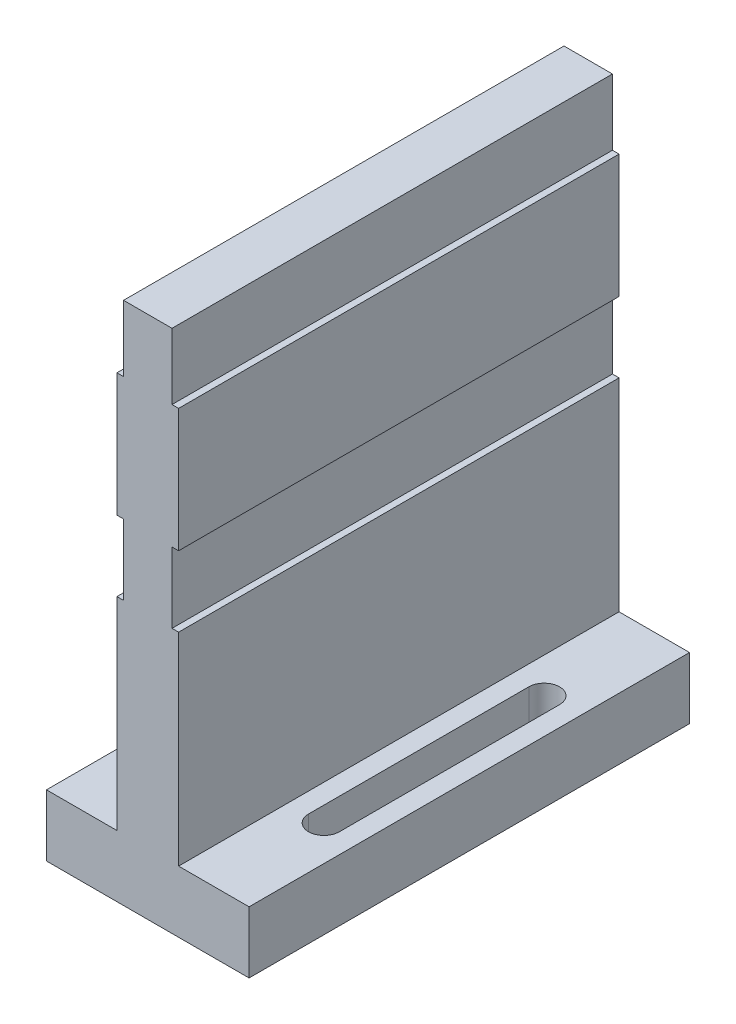
SolidWorks part; units mm, degrees
ref_plane "前视基准面" through (0, 0, 0) normal (0, 0, 1) x (1, 0, 0)
ref_plane "上视基准面" through (0, 0, 0) normal (0, 1, 0) x (1, 0, 0)
ref_plane "右视基准面" through (0, 0, 0) normal (1, 0, 0) x (0, 0, -1)
sketch "草图1" plane through (0, 0, 0) normal (0, 0, 1) x (1, 0, 0)
  line L0 (0, 0) -> (23, 0)
  line L1 (23, 0) -> (23, 14)
  line L2 (23, 14) -> (7, 14)
  line L3 (7, 14) -> (7, 119)
  line L4 (7, 119) -> (-7, 119)
  line L5 (-7, 119) -> (-7, 14)
  line L6 (-7, 14) -> (-23, 14)
  line L7 (-23, 14) -> (-23, 0)
  line L8 (-23, 0) -> (0, 0)
  dimension "D1" = 14
  dimension "D2" = 14
  dimension "D3" = 16
  dimension "D4" = 105
extrude "凸台-拉伸1" add sketch "草图1" along normal mid plane 100
sketch "草图2" plane through (0, 14, 0) normal (0, 1, 0) x (1, 0, 0)
  line L0 (15, -25) -> (15, 25) construction
  line L1 (11.5, -25) -> (11.5, 25)
  line L2 (18.5, -25) -> (18.5, 25)
  line L3 (23, -50) -> (23, 50) construction
  arc A0 (11.5, -25) -> (18.5, -25) centre (15, -25) ccw
  arc A1 (18.5, 25) -> (11.5, 25) centre (15, 25) ccw
  point P2 (15, 0)
  dimension "D3" = 3.5
  dimension "D1" = 50
  dimension "D2" = 8
extrude "切除-拉伸1" cut sketch "草图2" against normal up to next
sketch "草图3" plane through (7, 0, 0) normal (1, 0, 0) x (0, 0, -1)
  line L0 (50, 14) -> (50, 119) construction
  line L1 (-50, 119) -> (50, 119)
  line L2 (-50, 119) -> (-50, 104)
  line L3 (-50, 104) -> (50, 104)
  line L4 (50, 119) -> (50, 104)
  line L5 (-50, 14) -> (-50, 119) construction
  line L6 (-50, 76) -> (50, 76)
  line L7 (-50, 76) -> (-50, 60)
  line L8 (-50, 60) -> (50, 60)
  line L9 (50, 76) -> (50, 60)
  dimension "D1" = 15
  dimension "D2" = 16
  dimension "D3" = 28
extrude "切除-拉伸2" cut sketch "草图3" against normal blind 1.5
mirror "镜向1" about plane through (0, 0, 0) normal (1, 0, 0) of "切除-拉伸1"
mirror "镜向2" about plane through (0, 0, 0) normal (1, 0, 0) of "切除-拉伸2"
